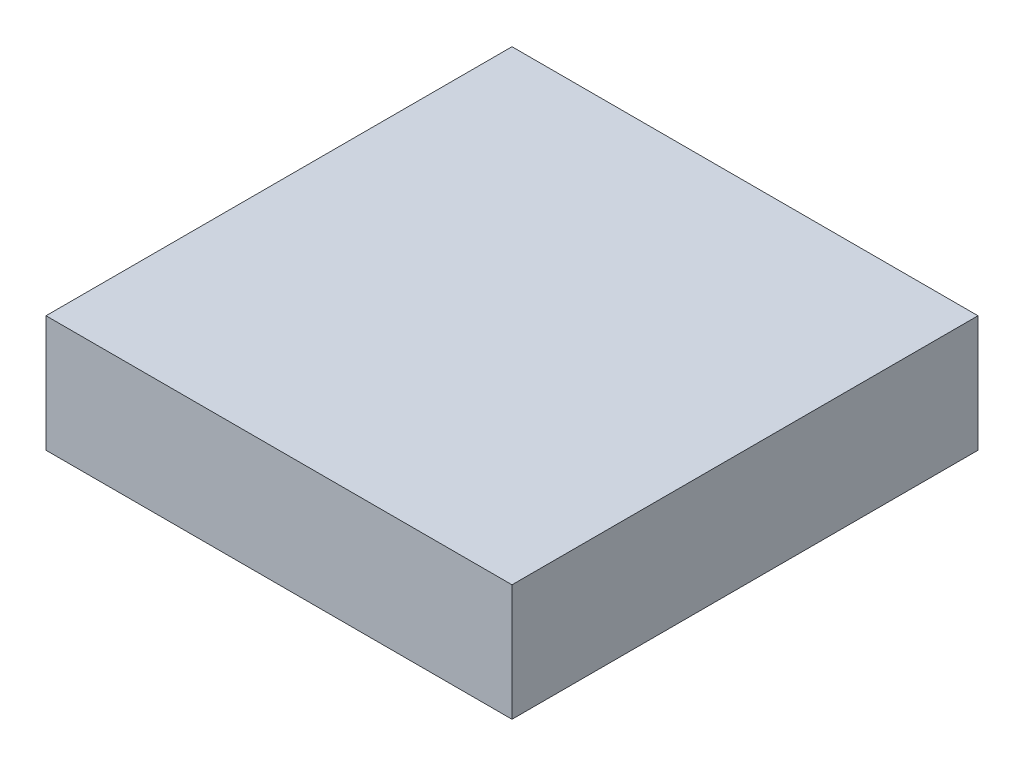
SolidWorks part; units mm, degrees
ref_plane "Front Plane" through (0, 0, 0) normal (0, 0, 1) x (1, 0, 0)
ref_plane "Top Plane" through (0, 0, 0) normal (0, 1, 0) x (1, 0, 0)
ref_plane "Right Plane" through (0, 0, 0) normal (1, 0, 0) x (0, 0, -1)
sketch "Sketch1" plane through (0, 0, 0) normal (0, 1, 0) x (1, 0, 0)
  line L1 (-4, 4) -> (4, 4)
  line L2 (-4, 4) -> (-4, -4)
  line L3 (-4, -4) -> (4, -4)
  line L4 (4, 4) -> (4, -4)
  line L5 (-4, 4) -> (4, -4) construction
  line L6 (-4, -4) -> (4, 4) construction
  point P0 (0, 0)
  dimension "D1" = 8
  dimension "D2" = 8
extrude "Boss-Extrude1" add sketch "Sketch1" along normal blind 2
